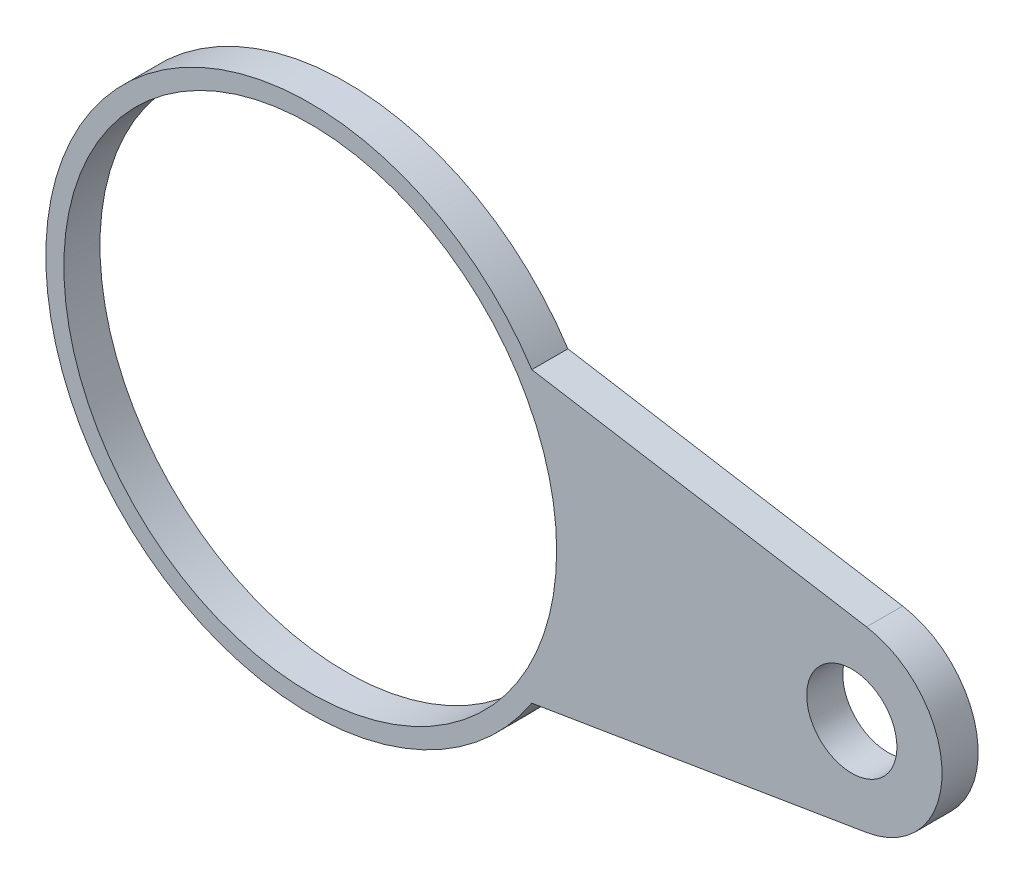
SolidWorks part; units mm, degrees
ref_plane "Front Plane" through (0, 0, 0) normal (0, 0, 1) x (1, 0, 0)
ref_plane "Top Plane" through (0, 0, 0) normal (0, 1, 0) x (1, 0, 0)
ref_plane "Right Plane" through (0, 0, 0) normal (1, 0, 0) x (0, 0, -1)
other "Configuration Table"
sketch "Sketch1" plane through (0, 0, 0) normal (0, 0, 1) x (1, 0, 0)
  line L0 (122.7284, 80) -> (308.1591, 49.3298)
  line L1 (0, 0) -> (300, 0) construction
  line L2 (122.7284, -80) -> (308.1591, -49.3298)
  arc A0 (122.7284, 80) -> (122.7284, -80) centre (0, 0) ccw
  arc A1 (308.1591, -49.3298) -> (308.1591, 49.3298) centre (300, 0) ccw
  circle A2 centre (300, 0) radius 25
  circle A3 centre (0, 0) radius 136.5
  dimension "D1" = 293
  dimension "D2" = 100
  dimension "D3" = 300
  dimension "D4" = 50
  dimension "D7" = 273
  dimension "D5" = 160
  dimension "D6" = 80
extrude "Boss-Extrude1" add sketch "Sketch1" along normal blind 20
